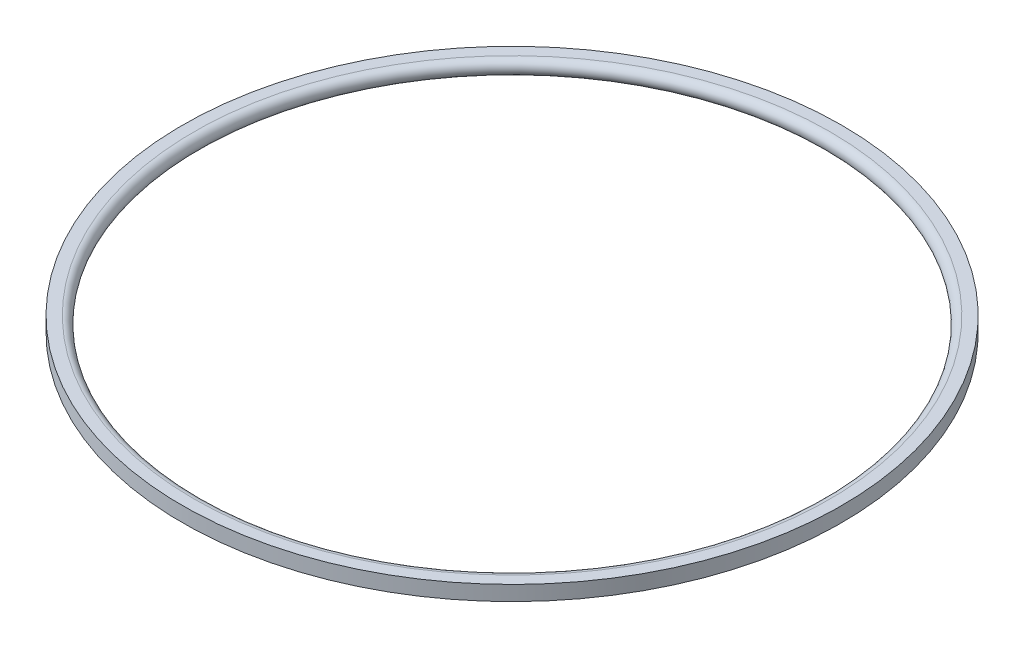
from build123d import *


with BuildPart() as part:
    # Sketch1 → Revolve1 (revolve)
    with BuildSketch(Plane.XY, mode=Mode.PRIVATE) as revolve1_sk:
        with BuildLine():
            Line((-171, 0), (-177.2, 0))
            Line((-177.2, 0), (-177.2, 8))
            Line((-177.2, 8), (-171, 8))
            ThreePointArc((-171, 8), (-167, 4), (-171, 0))
        make_face()
    revolve(revolve1_sk.sketch.rotate(Axis((0, 0, 0), (0, 1, 0)), 270), axis=Axis((0, 0, 0), (0, 1, 0)))


solid = part.part
